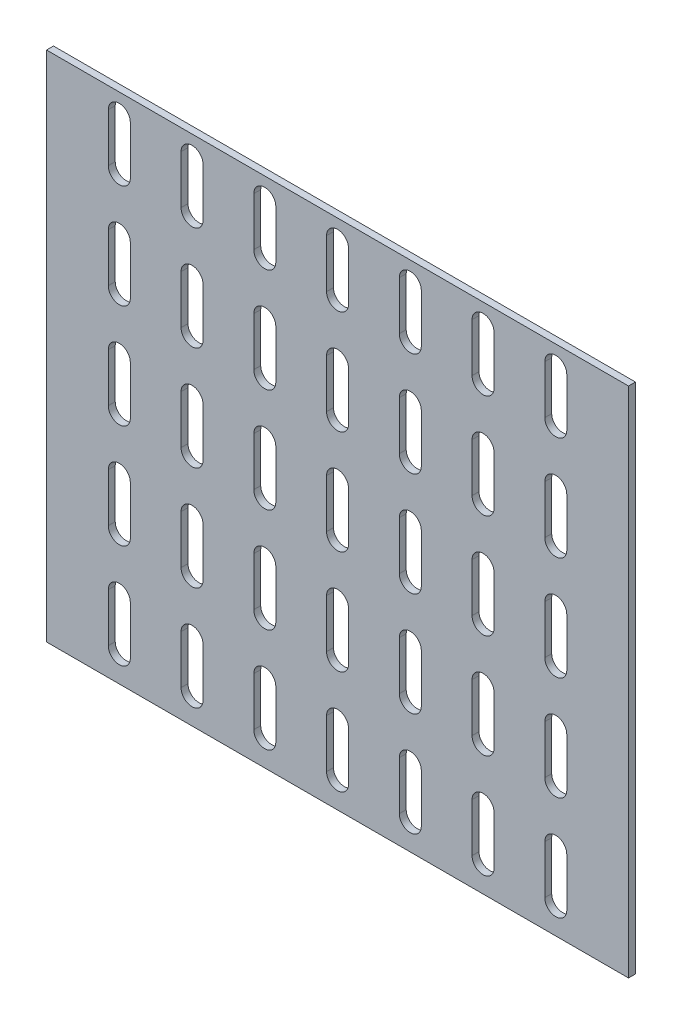
from build123d import *

# Parameters (mm, degrees)
SKETCH1_W           = 840
SKETCH1_H           = 740
BOSS_EXTRUDE1_DEPTH = 10
CUT_EXTRUDE1_DEPTH  = 10


with BuildPart() as part:
    # Sketch1 → Boss-Extrude1 (new body)
    with BuildSketch(Plane.XY):
        with Locations((368.938021937, -321.010102206)):
            Rectangle(SKETCH1_W, SKETCH1_H)
    extrude(amount=BOSS_EXTRUDE1_DEPTH)

    # Sketch2 → Cut-Extrude1 (cut)
    with BuildSketch(Plane.XY.offset(10)):
        with BuildLine():
            Line((69.818326735, 18.989897794), (69.818326735, -51.010102206))
            ThreePointArc((69.818326735, -51.010102206), (53.938021937, -66.890407004), (38.057717139, -51.010102206))
            Line((38.057717139, -51.010102206), (38.057717139, 18.989897794))
            ThreePointArc((38.057717139, 18.989897794), (53.938021937, 34.870202592), (69.818326735, 18.989897794))
        make_face()
        with BuildLine():
            Line((174.818326735, 18.989897794), (174.818326735, -51.010102206))
            ThreePointArc((174.818326735, -51.010102206), (158.938021937, -66.890407004), (143.057717139, -51.010102206))
            Line((143.057717139, -51.010102206), (143.057717139, 18.989897794))
            ThreePointArc((143.057717139, 18.989897794), (158.938021937, 34.870202592), (174.818326735, 18.989897794))
        make_face()
        with BuildLine():
            Line((279.818326735, 18.989897794), (279.818326735, -51.010102206))
            ThreePointArc((279.818326735, -51.010102206), (263.938021937, -66.890407004), (248.057717139, -51.010102206))
            Line((248.057717139, -51.010102206), (248.057717139, 18.989897794))
            ThreePointArc((248.057717139, 18.989897794), (263.938021937, 34.870202592), (279.818326735, 18.989897794))
        make_face()
        with BuildLine():
            Line((384.818326735, 18.989897794), (384.818326735, -51.010102206))
            ThreePointArc((384.818326735, -51.010102206), (368.938021937, -66.890407004), (353.057717139, -51.010102206))
            Line((353.057717139, -51.010102206), (353.057717139, 18.989897794))
            ThreePointArc((353.057717139, 18.989897794), (368.938021937, 34.870202592), (384.818326735, 18.989897794))
        make_face()
        with BuildLine():
            Line((489.818326735, 18.989897794), (489.818326735, -51.010102206))
            ThreePointArc((489.818326735, -51.010102206), (473.938021937, -66.890407004), (458.057717139, -51.010102206))
            Line((458.057717139, -51.010102206), (458.057717139, 18.989897794))
            ThreePointArc((458.057717139, 18.989897794), (473.938021937, 34.870202592), (489.818326735, 18.989897794))
        make_face()
        with BuildLine():
            Line((594.818326735, 18.989897794), (594.818326735, -51.010102206))
            ThreePointArc((594.818326735, -51.010102206), (578.938021937, -66.890407004), (563.057717139, -51.010102206))
            Line((563.057717139, -51.010102206), (563.057717139, 18.989897794))
            ThreePointArc((563.057717139, 18.989897794), (578.938021937, 34.870202592), (594.818326735, 18.989897794))
        make_face()
        with BuildLine():
            Line((699.818326735, 18.989897794), (699.818326735, -51.010102206))
            ThreePointArc((699.818326735, -51.010102206), (683.938021937, -66.890407004), (668.057717139, -51.010102206))
            Line((668.057717139, -51.010102206), (668.057717139, 18.989897794))
            ThreePointArc((668.057717139, 18.989897794), (683.938021937, 34.870202592), (699.818326735, 18.989897794))
        make_face()
        with BuildLine():
            Line((69.818326735, -131.010102206), (69.818326735, -201.010102206))
            ThreePointArc((69.818326735, -201.010102206), (53.938021937, -216.890407004), (38.057717139, -201.010102206))
            Line((38.057717139, -201.010102206), (38.057717139, -131.010102206))
            ThreePointArc((38.057717139, -131.010102206), (53.938021937, -115.129797408), (69.818326735, -131.010102206))
        make_face()
        with BuildLine():
            Line((174.818326735, -131.010102206), (174.818326735, -201.010102206))
            ThreePointArc((174.818326735, -201.010102206), (158.938021937, -216.890407004), (143.057717139, -201.010102206))
            Line((143.057717139, -201.010102206), (143.057717139, -131.010102206))
            ThreePointArc((143.057717139, -131.010102206), (158.938021937, -115.129797408), (174.818326735, -131.010102206))
        make_face()
        with BuildLine():
            Line((279.818326735, -131.010102206), (279.818326735, -201.010102206))
            ThreePointArc((279.818326735, -201.010102206), (263.938021937, -216.890407004), (248.057717139, -201.010102206))
            Line((248.057717139, -201.010102206), (248.057717139, -131.010102206))
            ThreePointArc((248.057717139, -131.010102206), (263.938021937, -115.129797408), (279.818326735, -131.010102206))
        make_face()
        with BuildLine():
            Line((384.818326735, -131.010102206), (384.818326735, -201.010102206))
            ThreePointArc((384.818326735, -201.010102206), (368.938021937, -216.890407004), (353.057717139, -201.010102206))
            Line((353.057717139, -201.010102206), (353.057717139, -131.010102206))
            ThreePointArc((353.057717139, -131.010102206), (368.938021937, -115.129797408), (384.818326735, -131.010102206))
        make_face()
        with BuildLine():
            Line((489.818326735, -131.010102206), (489.818326735, -201.010102206))
            ThreePointArc((489.818326735, -201.010102206), (473.938021937, -216.890407004), (458.057717139, -201.010102206))
            Line((458.057717139, -201.010102206), (458.057717139, -131.010102206))
            ThreePointArc((458.057717139, -131.010102206), (473.938021937, -115.129797408), (489.818326735, -131.010102206))
        make_face()
        with BuildLine():
            Line((594.818326735, -131.010102206), (594.818326735, -201.010102206))
            ThreePointArc((594.818326735, -201.010102206), (578.938021937, -216.890407004), (563.057717139, -201.010102206))
            Line((563.057717139, -201.010102206), (563.057717139, -131.010102206))
            ThreePointArc((563.057717139, -131.010102206), (578.938021937, -115.129797408), (594.818326735, -131.010102206))
        make_face()
        with BuildLine():
            Line((699.818326735, -131.010102206), (699.818326735, -201.010102206))
            ThreePointArc((699.818326735, -201.010102206), (683.938021937, -216.890407004), (668.057717139, -201.010102206))
            Line((668.057717139, -201.010102206), (668.057717139, -131.010102206))
            ThreePointArc((668.057717139, -131.010102206), (683.938021937, -115.129797408), (699.818326735, -131.010102206))
        make_face()
        with BuildLine():
            Line((69.818326735, -281.010102206), (69.818326735, -351.010102206))
            ThreePointArc((69.818326735, -351.010102206), (53.938021937, -366.890407004), (38.057717139, -351.010102206))
            Line((38.057717139, -351.010102206), (38.057717139, -281.010102206))
            ThreePointArc((38.057717139, -281.010102206), (53.938021937, -265.129797408), (69.818326735, -281.010102206))
        make_face()
        with BuildLine():
            Line((174.818326735, -281.010102206), (174.818326735, -351.010102206))
            ThreePointArc((174.818326735, -351.010102206), (158.938021937, -366.890407004), (143.057717139, -351.010102206))
            Line((143.057717139, -351.010102206), (143.057717139, -281.010102206))
            ThreePointArc((143.057717139, -281.010102206), (158.938021937, -265.129797408), (174.818326735, -281.010102206))
        make_face()
        with BuildLine():
            Line((279.818326735, -281.010102206), (279.818326735, -351.010102206))
            ThreePointArc((279.818326735, -351.010102206), (263.938021937, -366.890407004), (248.057717139, -351.010102206))
            Line((248.057717139, -351.010102206), (248.057717139, -281.010102206))
            ThreePointArc((248.057717139, -281.010102206), (263.938021937, -265.129797408), (279.818326735, -281.010102206))
        make_face()
        with BuildLine():
            Line((384.818326735, -281.010102206), (384.818326735, -351.010102206))
            ThreePointArc((384.818326735, -351.010102206), (368.938021937, -366.890407004), (353.057717139, -351.010102206))
            Line((353.057717139, -351.010102206), (353.057717139, -281.010102206))
            ThreePointArc((353.057717139, -281.010102206), (368.938021937, -265.129797408), (384.818326735, -281.010102206))
        make_face()
        with BuildLine():
            Line((489.818326735, -281.010102206), (489.818326735, -351.010102206))
            ThreePointArc((489.818326735, -351.010102206), (473.938021937, -366.890407004), (458.057717139, -351.010102206))
            Line((458.057717139, -351.010102206), (458.057717139, -281.010102206))
            ThreePointArc((458.057717139, -281.010102206), (473.938021937, -265.129797408), (489.818326735, -281.010102206))
        make_face()
        with BuildLine():
            Line((594.818326735, -281.010102206), (594.818326735, -351.010102206))
            ThreePointArc((594.818326735, -351.010102206), (578.938021937, -366.890407004), (563.057717139, -351.010102206))
            Line((563.057717139, -351.010102206), (563.057717139, -281.010102206))
            ThreePointArc((563.057717139, -281.010102206), (578.938021937, -265.129797408), (594.818326735, -281.010102206))
        make_face()
        with BuildLine():
            Line((699.818326735, -281.010102206), (699.818326735, -351.010102206))
            ThreePointArc((699.818326735, -351.010102206), (683.938021937, -366.890407004), (668.057717139, -351.010102206))
            Line((668.057717139, -351.010102206), (668.057717139, -281.010102206))
            ThreePointArc((668.057717139, -281.010102206), (683.938021937, -265.129797408), (699.818326735, -281.010102206))
        make_face()
        with BuildLine():
            Line((69.818326735, -431.010102206), (69.818326735, -501.010102206))
            ThreePointArc((69.818326735, -501.010102206), (53.938021937, -516.890407004), (38.057717139, -501.010102206))
            Line((38.057717139, -501.010102206), (38.057717139, -431.010102206))
            ThreePointArc((38.057717139, -431.010102206), (53.938021937, -415.129797408), (69.818326735, -431.010102206))
        make_face()
        with BuildLine():
            Line((174.818326735, -431.010102206), (174.818326735, -501.010102206))
            ThreePointArc((174.818326735, -501.010102206), (158.938021937, -516.890407004), (143.057717139, -501.010102206))
            Line((143.057717139, -501.010102206), (143.057717139, -431.010102206))
            ThreePointArc((143.057717139, -431.010102206), (158.938021937, -415.129797408), (174.818326735, -431.010102206))
        make_face()
        with BuildLine():
            Line((279.818326735, -431.010102206), (279.818326735, -501.010102206))
            ThreePointArc((279.818326735, -501.010102206), (263.938021937, -516.890407004), (248.057717139, -501.010102206))
            Line((248.057717139, -501.010102206), (248.057717139, -431.010102206))
            ThreePointArc((248.057717139, -431.010102206), (263.938021937, -415.129797408), (279.818326735, -431.010102206))
        make_face()
        with BuildLine():
            Line((384.818326735, -431.010102206), (384.818326735, -501.010102206))
            ThreePointArc((384.818326735, -501.010102206), (368.938021937, -516.890407004), (353.057717139, -501.010102206))
            Line((353.057717139, -501.010102206), (353.057717139, -431.010102206))
            ThreePointArc((353.057717139, -431.010102206), (368.938021937, -415.129797408), (384.818326735, -431.010102206))
        make_face()
        with BuildLine():
            Line((489.818326735, -431.010102206), (489.818326735, -501.010102206))
            ThreePointArc((489.818326735, -501.010102206), (473.938021937, -516.890407004), (458.057717139, -501.010102206))
            Line((458.057717139, -501.010102206), (458.057717139, -431.010102206))
            ThreePointArc((458.057717139, -431.010102206), (473.938021937, -415.129797408), (489.818326735, -431.010102206))
        make_face()
        with BuildLine():
            Line((594.818326735, -431.010102206), (594.818326735, -501.010102206))
            ThreePointArc((594.818326735, -501.010102206), (578.938021937, -516.890407004), (563.057717139, -501.010102206))
            Line((563.057717139, -501.010102206), (563.057717139, -431.010102206))
            ThreePointArc((563.057717139, -431.010102206), (578.938021937, -415.129797408), (594.818326735, -431.010102206))
        make_face()
        with BuildLine():
            Line((699.818326735, -431.010102206), (699.818326735, -501.010102206))
            ThreePointArc((699.818326735, -501.010102206), (683.938021937, -516.890407004), (668.057717139, -501.010102206))
            Line((668.057717139, -501.010102206), (668.057717139, -431.010102206))
            ThreePointArc((668.057717139, -431.010102206), (683.938021937, -415.129797408), (699.818326735, -431.010102206))
        make_face()
        with BuildLine():
            Line((69.818326735, -581.010102206), (69.818326735, -651.010102206))
            ThreePointArc((69.818326735, -651.010102206), (53.938021937, -666.890407004), (38.057717139, -651.010102206))
            Line((38.057717139, -651.010102206), (38.057717139, -581.010102206))
            ThreePointArc((38.057717139, -581.010102206), (53.938021937, -565.129797408), (69.818326735, -581.010102206))
        make_face()
        with BuildLine():
            Line((174.818326735, -581.010102206), (174.818326735, -651.010102206))
            ThreePointArc((174.818326735, -651.010102206), (158.938021937, -666.890407004), (143.057717139, -651.010102206))
            Line((143.057717139, -651.010102206), (143.057717139, -581.010102206))
            ThreePointArc((143.057717139, -581.010102206), (158.938021937, -565.129797408), (174.818326735, -581.010102206))
        make_face()
        with BuildLine():
            Line((279.818326735, -581.010102206), (279.818326735, -651.010102206))
            ThreePointArc((279.818326735, -651.010102206), (263.938021937, -666.890407004), (248.057717139, -651.010102206))
            Line((248.057717139, -651.010102206), (248.057717139, -581.010102206))
            ThreePointArc((248.057717139, -581.010102206), (263.938021937, -565.129797408), (279.818326735, -581.010102206))
        make_face()
        with BuildLine():
            Line((384.818326735, -581.010102206), (384.818326735, -651.010102206))
            ThreePointArc((384.818326735, -651.010102206), (368.938021937, -666.890407004), (353.057717139, -651.010102206))
            Line((353.057717139, -651.010102206), (353.057717139, -581.010102206))
            ThreePointArc((353.057717139, -581.010102206), (368.938021937, -565.129797408), (384.818326735, -581.010102206))
        make_face()
        with BuildLine():
            Line((489.818326735, -581.010102206), (489.818326735, -651.010102206))
            ThreePointArc((489.818326735, -651.010102206), (473.938021937, -666.890407004), (458.057717139, -651.010102206))
            Line((458.057717139, -651.010102206), (458.057717139, -581.010102206))
            ThreePointArc((458.057717139, -581.010102206), (473.938021937, -565.129797408), (489.818326735, -581.010102206))
        make_face()
        with BuildLine():
            Line((594.818326735, -581.010102206), (594.818326735, -651.010102206))
            ThreePointArc((594.818326735, -651.010102206), (578.938021937, -666.890407004), (563.057717139, -651.010102206))
            Line((563.057717139, -651.010102206), (563.057717139, -581.010102206))
            ThreePointArc((563.057717139, -581.010102206), (578.938021937, -565.129797408), (594.818326735, -581.010102206))
        make_face()
        with BuildLine():
            Line((699.818326735, -581.010102206), (699.818326735, -651.010102206))
            ThreePointArc((699.818326735, -651.010102206), (683.938021937, -666.890407004), (668.057717139, -651.010102206))
            Line((668.057717139, -651.010102206), (668.057717139, -581.010102206))
            ThreePointArc((668.057717139, -581.010102206), (683.938021937, -565.129797408), (699.818326735, -581.010102206))
        make_face()
    extrude(amount=-CUT_EXTRUDE1_DEPTH, mode=Mode.SUBTRACT)


solid = part.part
